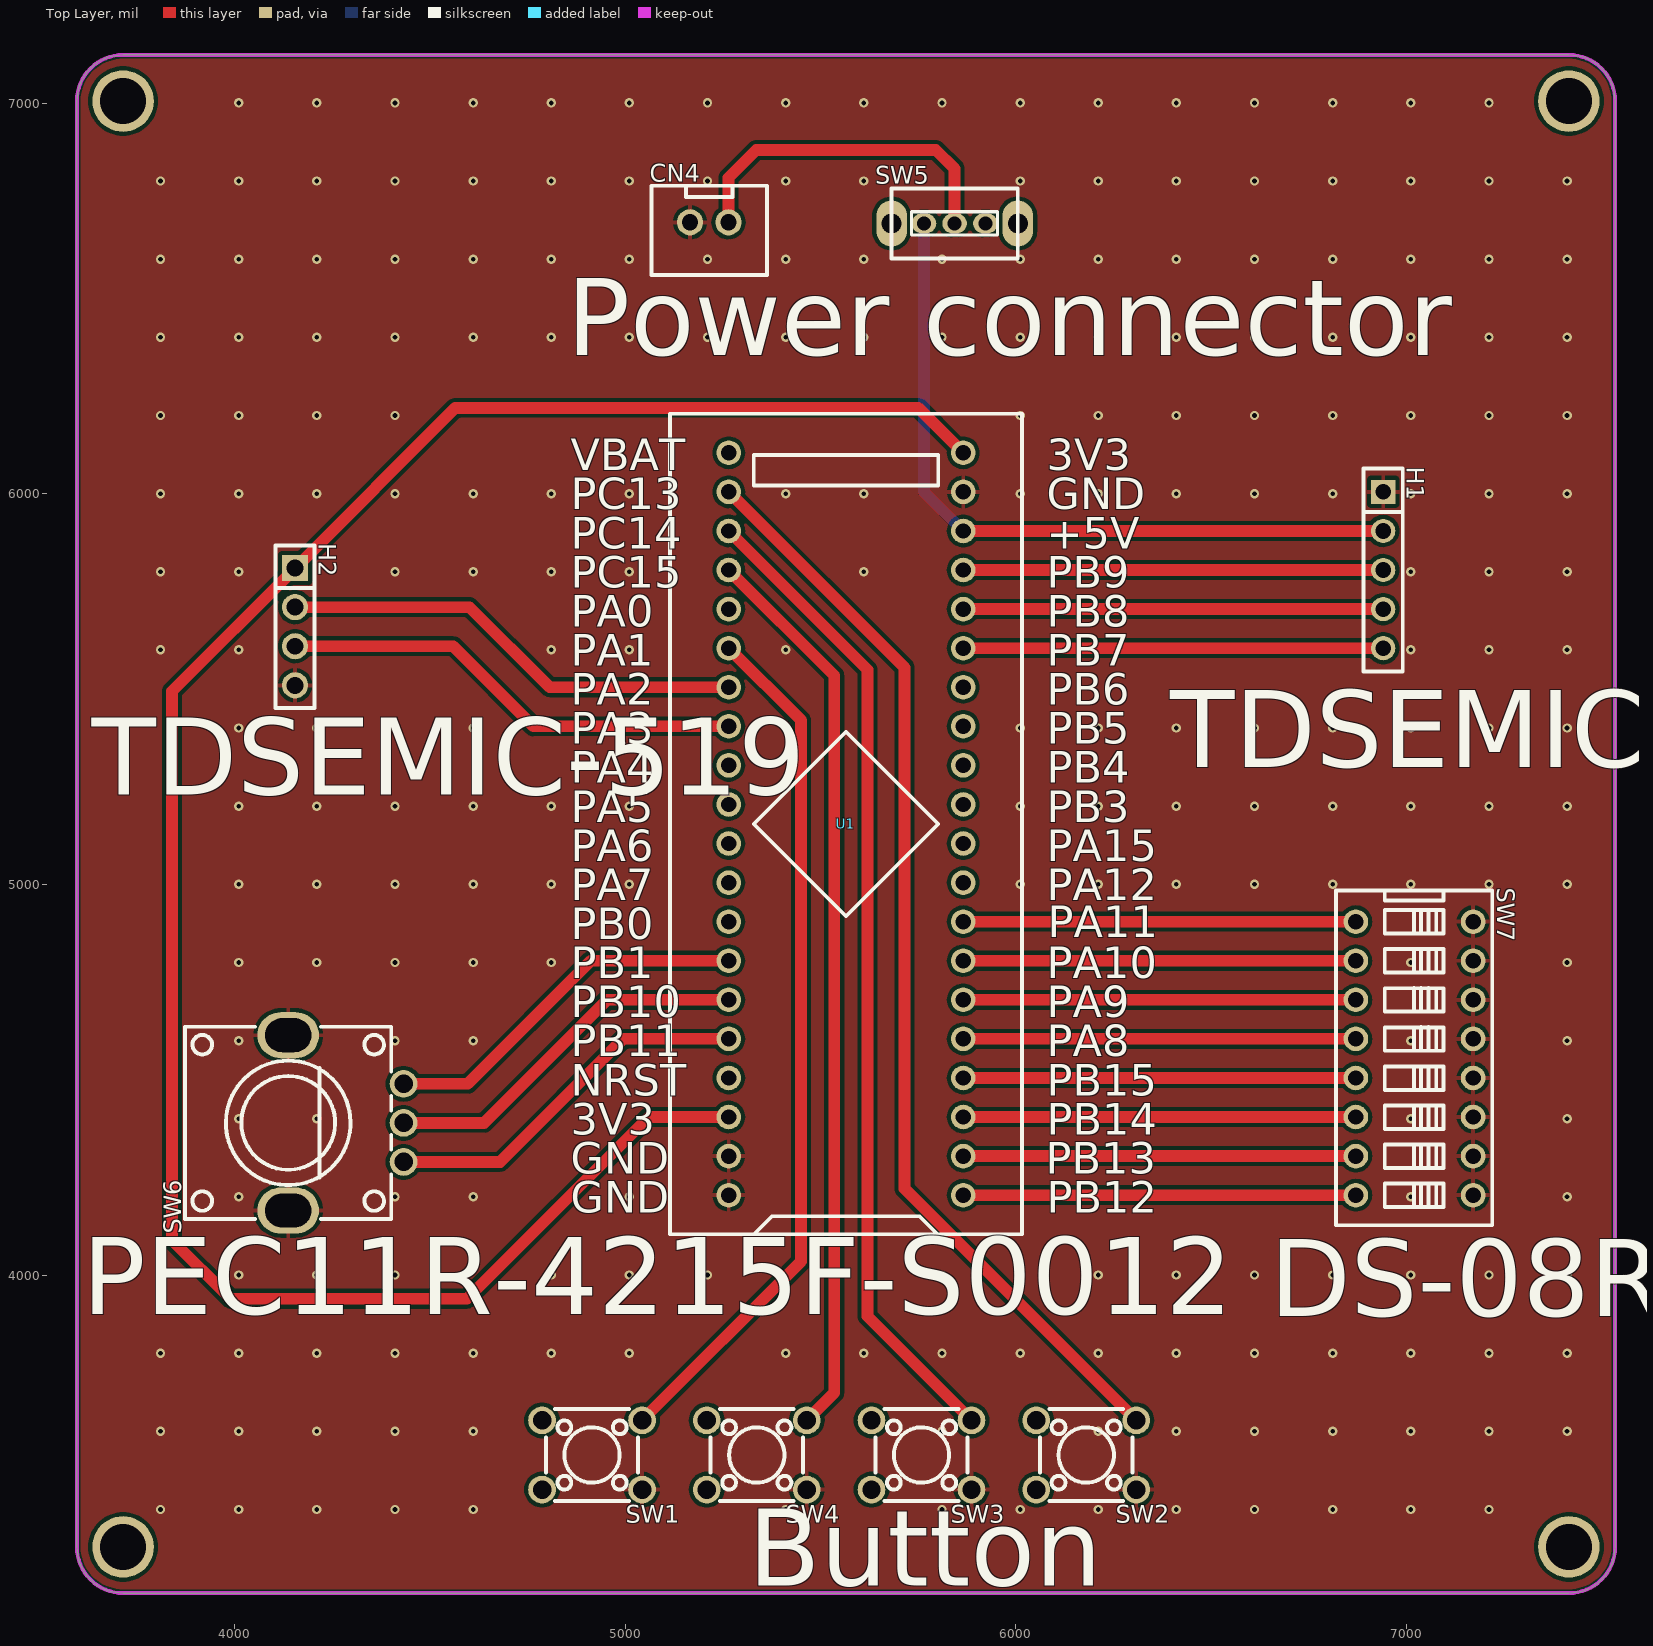
[diagram p0: Top Layer view]
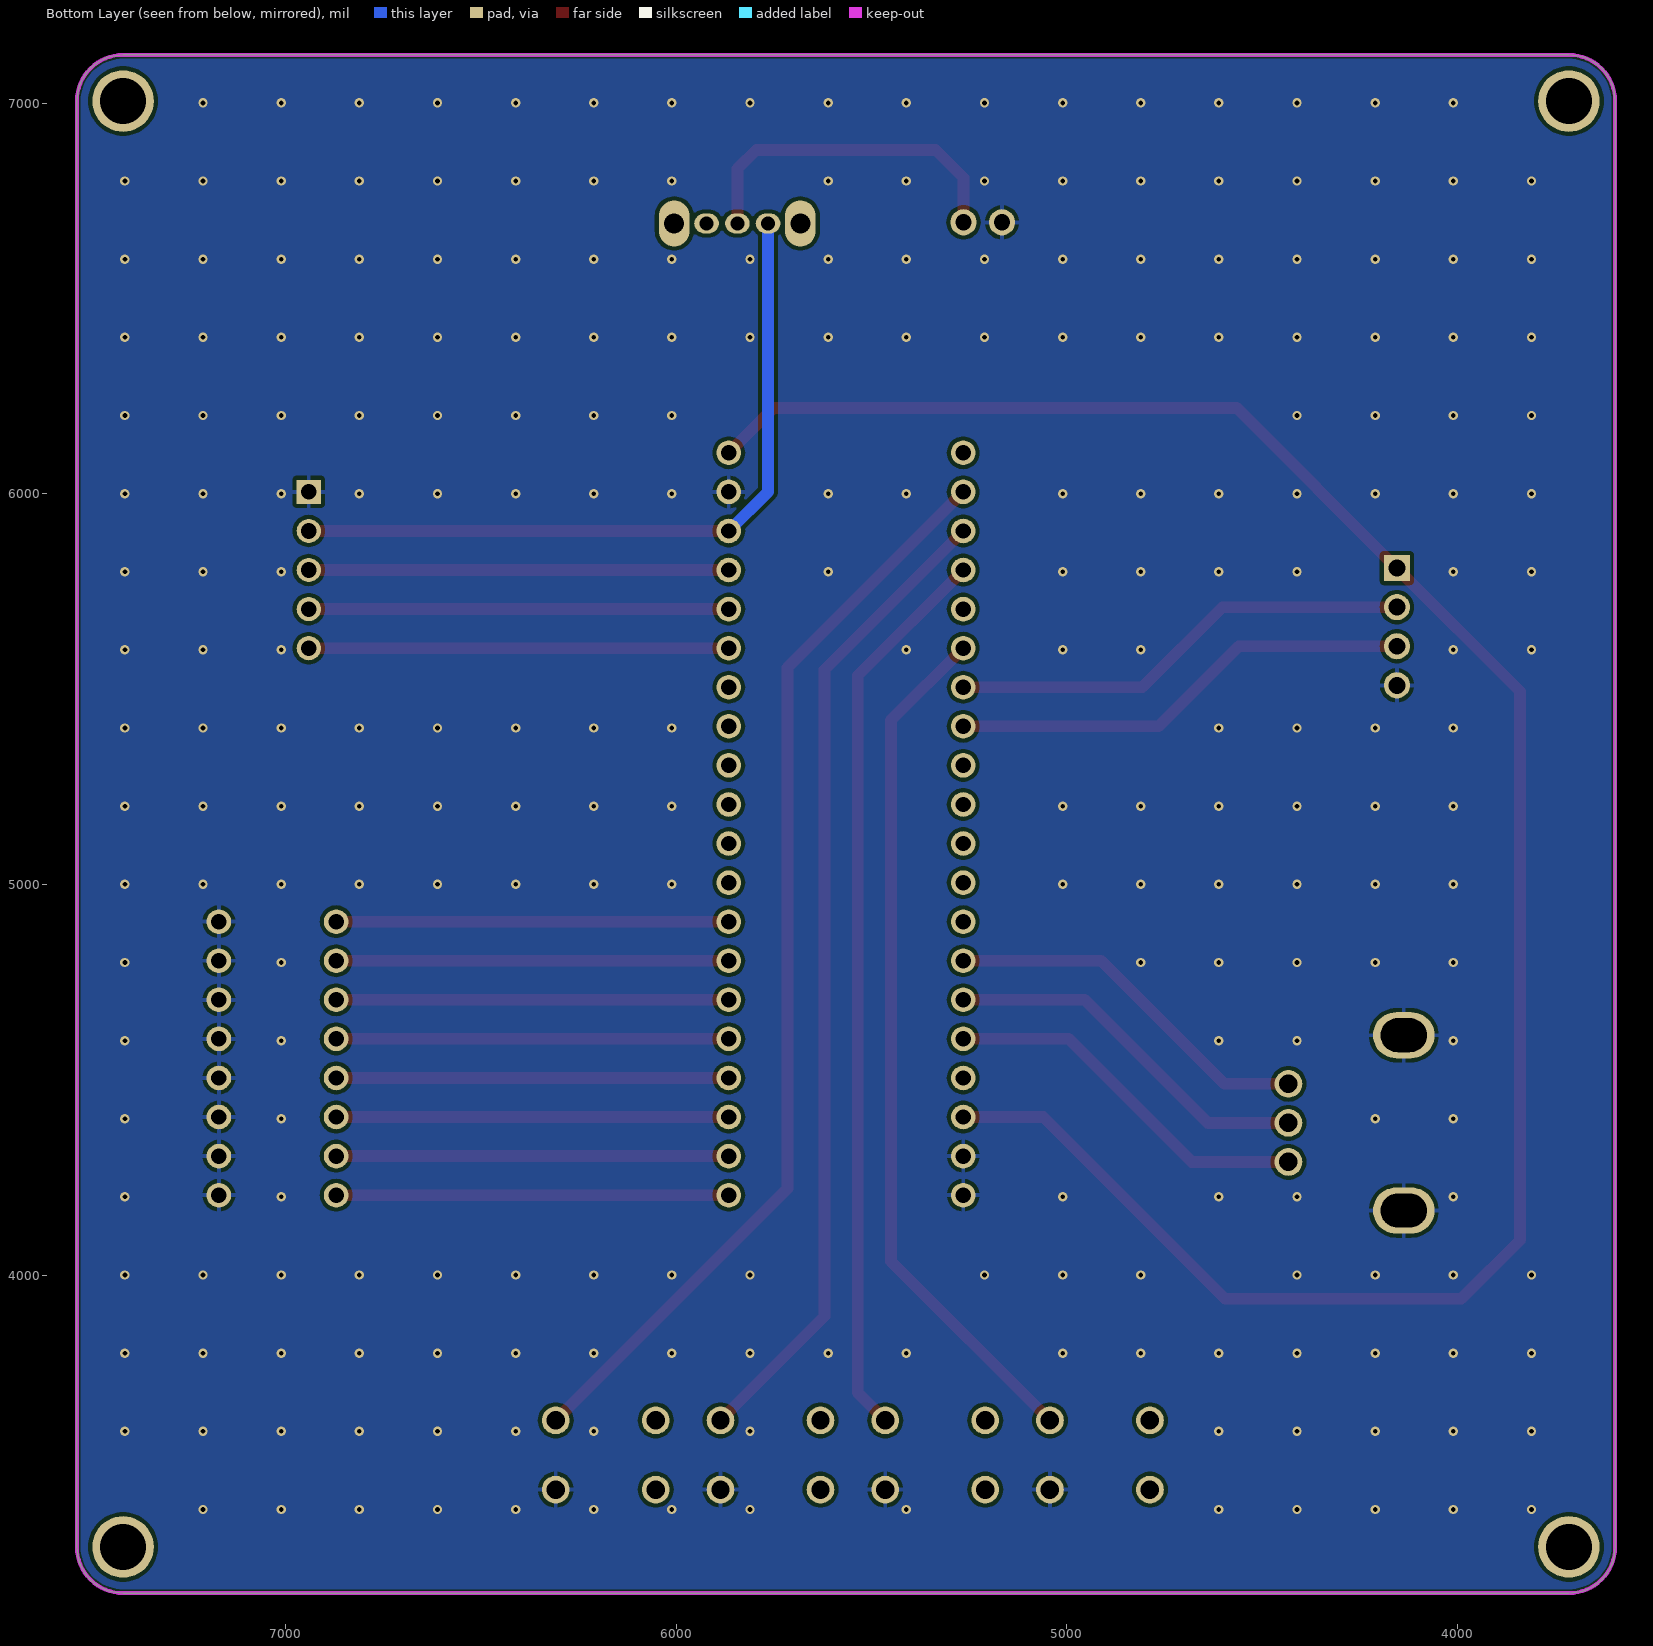
[diagram p1: Bottom Layer view, seen from below]
# Altium PCB MISC51872.pcbdoc
Units mil, origin at the board's own origin, x right, y up, seen from the top; angles counter-clockwise.
Board outline 3937.01 x 3937.01 mil, 2 copper layers (Top Layer, Bottom Layer), stack 62.206 mil thick; 11 components, 38 nets, 97 pads, 243 vias.

## Layer stack, top to bottom
Top Solder Mask Layer: solder mask 0.394, Dk 3.3
Top Layer: signal copper 1.379
Dielectric1: surface 59.449, FR4, Dk 4.5
Bottom Layer: signal copper 1.378
Bottom Solder Mask Layer: solder mask 0.394, Dk 3.3

## Board outline
3714.61,7123.5 ccw(c3714.61,7005.39) 3596.5,7005.39 3596.5,3304.61 ccw(c3714.61,3304.61) 3714.61,3186.5 7415.39,3186.5 ccw(c7415.39,3304.61) 7533.5,3304.61 7533.5,7005.39 ccw(c7415.39,7005.39) 7415.39,7123.5 3714.61,7123.5

## Design rules (kind name [scope] priority, off if disabled: settings)
BoardOutlineClearance copperThickness2oz_1 [All] p2 off: genericclearance=7.99 ignorepadtopadclearanceinfootprint=FALSE except(0: Arc-SplitContinuation Track-SplitContinuation SMDPad-SplitContinuation THPad-SplitContinuation Via-SplitContinuation Fill-SplitContinuation Region-SplitContinuation Poly-SplitContinuation Text-SplitContinuation Hole-SplitContinuation; 5.98: Arc-CutoutEdge Track-CutoutEdge SMDPad-CutoutEdge THPad-CutoutEdge Via-CutoutEdge Text-CutoutEdge; 6.9: Hole-OutlineEdge Hole-CutoutEdge; 10: Poly-OutlineEdge Poly-CutoutEdge; 11.81: Arc-OutlineEdge Track-OutlineEdge SMDPad-OutlineEdge THPad-OutlineEdge Via-OutlineEdge Fill-OutlineEdge Region-OutlineEdge Text-OutlineEdge Fill-CutoutEdge Region-CutoutEdge)
BoardOutlineClearance Plane_innerPlane_1 [All] p4 off: genericclearance=4.02 ignorepadtopadclearanceinfootprint=FALSE except(0: Arc-SplitContinuation Track-SplitContinuation SMDPad-SplitContinuation THPad-SplitContinuation Via-SplitContinuation Fill-SplitContinuation Region-SplitContinuation Poly-SplitContinuation Text-SplitContinuation Hole-SplitContinuation; 5.98: Arc-CutoutEdge Track-CutoutEdge SMDPad-CutoutEdge THPad-CutoutEdge Via-CutoutEdge Text-CutoutEdge; 6.9: Hole-OutlineEdge Hole-CutoutEdge; 10: Poly-OutlineEdge Poly-CutoutEdge; 11.81: Arc-OutlineEdge Track-OutlineEdge SMDPad-OutlineEdge THPad-OutlineEdge Via-OutlineEdge Fill-OutlineEdge Region-OutlineEdge Text-OutlineEdge Fill-CutoutEdge Region-CutoutEdge)
BoardOutlineClearance Copper_copperRegion_1 [All] p6 off: genericclearance=4.02 ignorepadtopadclearanceinfootprint=FALSE except(0: Arc-SplitContinuation Track-SplitContinuation SMDPad-SplitContinuation THPad-SplitContinuation Via-SplitContinuation Fill-SplitContinuation Region-SplitContinuation Poly-SplitContinuation Text-SplitContinuation Hole-SplitContinuation; 5.98: Arc-CutoutEdge Track-CutoutEdge SMDPad-CutoutEdge THPad-CutoutEdge Via-CutoutEdge Text-CutoutEdge; 6.9: Hole-OutlineEdge Hole-CutoutEdge; 10: Poly-OutlineEdge Poly-CutoutEdge; 11.81: Arc-OutlineEdge Track-OutlineEdge SMDPad-OutlineEdge THPad-OutlineEdge Via-OutlineEdge Fill-OutlineEdge Region-OutlineEdge Text-OutlineEdge Fill-CutoutEdge Region-CutoutEdge)
BoardOutlineClearance copperThickness1oz_1 [All] p8: genericclearance=4.02 ignorepadtopadclearanceinfootprint=FALSE except(0: Arc-SplitContinuation Track-SplitContinuation SMDPad-SplitContinuation THPad-SplitContinuation Via-SplitContinuation Fill-SplitContinuation Region-SplitContinuation Poly-SplitContinuation Text-SplitContinuation Hole-SplitContinuation; 5.98: Arc-CutoutEdge Track-CutoutEdge SMDPad-CutoutEdge THPad-CutoutEdge Via-CutoutEdge Text-CutoutEdge; 6.9: Hole-OutlineEdge Hole-CutoutEdge; 10: Poly-OutlineEdge Poly-CutoutEdge; 11.81: Arc-OutlineEdge Track-OutlineEdge SMDPad-OutlineEdge THPad-OutlineEdge Via-OutlineEdge Fill-OutlineEdge Region-OutlineEdge Text-OutlineEdge Fill-CutoutEdge Region-CutoutEdge)
Clearance copperThickness2oz [All] p1 off: gap=7.99 ignorepadtopadclearanceinfootprint=FALSE except(5.98: SMDPad-Track SMDPad-SMDPad THPad-Track SMDPad-THPad THPad-THPad Track-Via SMDPad-Via THPad-Via Via-Via Fill-SMDPad Region-SMDPad Fill-THPad Region-THPad Fill-Via Region-Via Fill-Fill Fill-Region Region-Region Arc-Track Arc-SMDPad Arc-THPad Arc-Via Fill-Arc Region-Arc Arc-Arc Text-Track SMDPad-Text Text-THPad Text-Via Fill-Text Region-Text Arc-Text Text-Text; 6.9: Hole-Track Hole-SMDPad Hole-THPad Hole-Via Fill-Hole Region-Hole Hole-Arc Hole-Text; 10: Poly-Track Poly-SMDPad Poly-THPad Poly-Via Poly-Fill Poly-Region Poly-Poly Poly-Arc Poly-Text Poly-Hole; 11.81: Fill-Track Region-Track)
Clearance Plane_innerPlane [All] p3 off: gap=4.02 ignorepadtopadclearanceinfootprint=FALSE except(5.98: SMDPad-Track SMDPad-SMDPad THPad-Track SMDPad-THPad THPad-THPad Track-Via SMDPad-Via THPad-Via Via-Via Fill-SMDPad Region-SMDPad Fill-THPad Region-THPad Fill-Via Region-Via Fill-Fill Fill-Region Region-Region Arc-Track Arc-SMDPad Arc-THPad Arc-Via Fill-Arc Region-Arc Arc-Arc Text-Track SMDPad-Text Text-THPad Text-Via Fill-Text Region-Text Arc-Text Text-Text; 6.9: Hole-Track Hole-SMDPad Hole-THPad Hole-Via Fill-Hole Region-Hole Hole-Arc Hole-Text; 10: Poly-Track Poly-SMDPad Poly-THPad Poly-Via Poly-Fill Poly-Region Poly-Poly Poly-Arc Poly-Text Poly-Hole; 11.81: Fill-Track Region-Track)
Clearance Copper_copperRegion [All] p5 off: gap=4.02 ignorepadtopadclearanceinfootprint=FALSE except(5.98: SMDPad-Track SMDPad-SMDPad THPad-Track SMDPad-THPad THPad-THPad Track-Via SMDPad-Via THPad-Via Via-Via Fill-SMDPad Region-SMDPad Fill-THPad Region-THPad Fill-Via Region-Via Fill-Fill Fill-Region Region-Region Arc-Track Arc-SMDPad Arc-THPad Arc-Via Fill-Arc Region-Arc Arc-Arc Text-Track SMDPad-Text Text-THPad Text-Via Fill-Text Region-Text Arc-Text Text-Text; 6.9: Hole-Track Hole-SMDPad Hole-THPad Hole-Via Fill-Hole Region-Hole Hole-Arc Hole-Text; 10: Poly-Track Poly-SMDPad Poly-THPad Poly-Via Poly-Fill Poly-Region Poly-Poly Poly-Arc Poly-Text Poly-Hole; 11.81: Fill-Track Region-Track)
Clearance copperThickness1oz [All] p7: gap=4.02 ignorepadtopadclearanceinfootprint=FALSE except(5.98: SMDPad-Track SMDPad-SMDPad THPad-Track SMDPad-THPad THPad-THPad Track-Via SMDPad-Via THPad-Via Via-Via Fill-SMDPad Region-SMDPad Fill-THPad Region-THPad Fill-Via Region-Via Fill-Fill Fill-Region Region-Region Arc-Track Arc-SMDPad Arc-THPad Arc-Via Fill-Arc Region-Arc Arc-Arc Text-Track SMDPad-Text Text-THPad Text-Via Fill-Text Region-Text Arc-Text Text-Text; 6.9: Hole-Track Hole-SMDPad Hole-THPad Hole-Via Fill-Hole Region-Hole Hole-Arc Hole-Text; 10: Poly-Track Poly-SMDPad Poly-THPad Poly-Via Poly-Fill Poly-Region Poly-Poly Poly-Arc Poly-Text Poly-Hole; 11.81: Fill-Track Region-Track)
DiffPairsRouting differentialPair [All] p1: maxlimit=6 minlimit=6 mostfreqgap=6 toplayer_minwidth=5 toplayer_prefwidth=10 toplayer_maxwidth=100 toplayer_mingap=6 toplayer_prefgap=6 toplayer_maxgap=6 bottomlayer_minwidth=5 bottomlayer_prefwidth=10 bottomlayer_maxwidth=100 bottomlayer_mingap=6 bottomlayer_prefgap=6 bottomlayer_maxgap=6 maxuncoupledlength=10
HoleToHoleClearance otherClearance [All] p1: gap=11.81 allowstackedmicrovias=TRUE
Length netLength [All] p1: minlimit=0 maxlimit=0
PasteMaskExpansion pasteMaskExpansion [All] p1: expansion=0
PlaneConnect innerPlane [All] p1: planeconnectstyle=Relief reliefexpansion=20 reliefentries=4 reliefconductorwidth=10 reliefairgap=10
PolygonConnect copperRegion [All] p1: connectstyle=Relief reliefconductorwidth=10 reliefentries=4 polygonreliefangle="90 Angle" airgapwidth=10 via.connectstyle=Relief via.reliefconductorwidth=10 via.reliefentries=4 via.polygonreliefangle="90 Angle" via.airgapwidth=10
RoutingVias viaSize [All] p1: holewidth=12.01 width=24.02 viastyle="Through Hole" minholewidth=11.81 minwidth=19.68 maxholewidth=248.03 maxwidth=393.7
SolderMaskExpansion solderMaskExpansion [IsVia] p1: expansion=-1000 istentingtop=TRUE
SolderMaskExpansion solderMaskExpansion [All] p2: expansion=2 istentingtop=FALSE
Width copperThickness2oz_2 [All] p1 off: maxlimit=100 minlimit=8 preferedwidth=10
Width copperThickness1oz_2 [All] p2: maxlimit=100 minlimit=5 preferedwidth=10

## Components (designator, comment, footprint, x,y, rotation, side; value= is the part's Value field where it differs from the comment)
CN4 "XH2.54*2P_THT" CONN-TH_2P-P2.50-XH2.54-2P 5215,6695 r0 top
H1 "" HDR-TH_5P-P2.54-V-F 6940,5805 r270 top
H2 "" HDR-TH_4P-P2.54-V-F 4155,5660 r270 top
SW1 "" SW-TH_4P-L6.0-W6.0-P4.50-LS6.5 4915,3540 r180 top
SW2 "" SW-TH_4P-L6.0-W6.0-P4.50-LS6.5 6179.9,3540 r180 top
SW3 "" SW-TH_4P-L6.0-W6.0-P4.50-LS6.5 5758.27,3540 r180 top
SW4 "" SW-TH_4P-L6.0-W6.0-P4.50-LS6.5 5336.63,3540 r180 top
SW5 "" 拨动开关 5837.9,6692.05 r0 top
SW6 "PEC11R-4215F-N0024" SW-TH_PEC11R-4215F-N0024 4285,4390 r90 top
SW7 "DS-08RP" SW-TH_DS-08XP 7020,4555 r270 top
U1 "STM32F103C8T6-Card" CONN-TH_L53.3-W22.9_STM32F103C8T6-CARD 5565,5155 r90 top

## Footprints (in the part's own frame and the unit in brackets; to place one, negate y for a bottom-side part, rotate by r counter-clockwise, add the part's x,y. Pads: shape width x height; smd on the part's side, far side on the other; paste and mask are expansions set on the pad)
CONN-TH_2P-P2.50-XH2.54-2P [mm]
  round 1.7 hole 1.05 paste+0 mask+0.05: 1(1.25,0) 2(-1.25,0)
  silkscreen extent -3.75,-3.42 3.75,2.37
CONN-TH_L53.3-W22.9_STM32F103C8T6-CARD [mm]
  round 1.6 hole 1: 1(-24.13,-7.62) 2(-21.59,-7.62) 3(-19.05,-7.62) 4(-16.51,-7.62) 5(-13.97,-7.62) 6(-11.43,-7.62) 7(-8.89,-7.62) 8(-6.35,-7.62) 9(-3.81,-7.62) 10(-1.27,-7.62) 11(1.27,-7.62) 12(3.81,-7.62) 13(6.35,-7.62) 14(8.89,-7.62) 15(11.43,-7.62) 16(13.97,-7.62) 17(16.51,-7.62) 18(19.05,-7.62) 19(21.59,-7.62) 20(24.13,-7.62) 21(24.13,7.62) 22(21.59,7.62) 23(19.05,7.62) 24(16.51,7.62) 25(13.97,7.62) 26(11.43,7.62) 27(8.89,7.62) 28(6.35,7.62) 29(3.81,7.62) 30(1.27,7.62) 31(-1.27,7.62) 32(-3.81,7.62) 33(-6.35,7.62) 34(-8.89,7.62) 35(-11.43,7.62) 36(-13.97,7.62) 37(-16.51,7.62) 38(-19.05,7.62) 39(-21.59,7.62) 40(-24.13,7.62)
  silkscreen extent -26.67,-11.43 26.67,11.43
HDR-TH_4P-P2.54-V-F [mm]
  rect 1.7x1.7 hole 1.1: 1(-3.81,0)
  round 1.7 hole 1.1: 2(-1.27,0) 3(1.27,0) 4(3.81,0)
  silkscreen extent -5.29,-1.27 5.29,1.27
HDR-TH_5P-P2.54-V-F [mil]
  rect 62x62 hole 40.16: 1(-200,0)
  round 62 hole 40.16: 2(-100,0) 3(0,0) 4(100,0) 5(200,0)
  silkscreen extent -260,-50 260,50
SW-TH_4P-L6.0-W6.0-P4.50-LS6.5 [mm]
  round 1.8 hole 1.2: 1(-3.25,2.25) 2(3.25,2.25) 3(-3.25,-2.25) 4(3.25,-2.25)
  silkscreen extent -3,-3 3,3
SW-TH_DS-08XP [mm]
  round 1.6 hole 1: 1(-8.89,3.81) 2(-6.35,3.81) 3(-3.81,3.81) 4(-1.27,3.81) 5(1.27,3.81) 6(3.81,3.81) 7(6.35,3.81) 8(8.89,3.81) 9(8.89,-3.81) 10(6.35,-3.81) 11(3.81,-3.81) 12(1.27,-3.81) 13(-1.27,-3.81) 14(-3.81,-3.81) 15(-6.35,-3.81) 16(-8.89,-3.81)
  silkscreen extent -10.91,-5.11 10.85,5.05
SW-TH_PEC11R-4215F-N0024 [mm]
  oval 3x4 hole 2.2 slot 3 at 90 deg: 4(-5.7,3.75) 5(5.7,3.75)
  round 1.8 hole 1.2: A(-2.54,-3.75) B(2.54,-3.75) C(0,-3.75)
  silkscreen extent -6.25,-2.95 6.25,10.45
拨动开关 [mil]
  oval 63x51.2 hole 35.4 paste+0 mask+2: 1(-73.4,0) 2(5,0) 3(84,0)
  oval 78.7x118.1 hole 51.2 paste+0 mask+2: 4(166.7,0) 5(-156.1,0)
  silkscreen extent -156,-90 167,90

## Free pads (board coordinates)
  round 157.48 hole 118.11: 1(3714.61,7005.39) 1(3714.61,3304.61) 1(7415.39,7005.39) 1(7415.39,3304.61)

## Via types
v1: diameter 24.02, hole 12, Top Layer to Bottom Layer, 243 vias

## Nets (pads, with @x,y where several pads share a name; then routed paths per layer and width w, separated by ;. In a path a pad name is that pad's centre, name@x,y a point inside that pad or via, vN(x,y) a via of type N, cw(c..) or ccw(c..) an arc to the next point about the centre after c; other vN are vias at no path point)
$1N17118: CN4.1 SW5.2 | length 882.1
  Top Layer w30: CN4.1 5264.22,6809.22 5335,6880 5795,6880 5842.9,6832.1 SW5.2
+5V: H1.2 SW5.1 U1.18 | length 1903.7
  Top Layer w30: U1.18 H1.2
  Bottom Layer w30: SW5.1 5764.5,6005.5 U1.18
GND: CN4.2 H1.1 H2.4 SW1.1 SW2.1 SW3.1 SW4.1 SW6.4 SW6.5 SW7.1 SW7.2 SW7.3 SW7.4 SW7.5 SW7.6 SW7.7 SW7.8 U1.19 U1.39 U1.40
  other v1: 3810.6,3400.6 4010.6,3400.6 4210.6,3400.6 4410.6,3400.6 4610.6,3400.6 5410.6,3400.6 5810.6,3400.6 6010.6,3400.6 6210.6,3400.6 6410.6,3400.6 6610.6,3400.6 6810.6,3400.6 7010.6,3400.6 7210.6,3400.6 3810.6,3600.6 4010.6,3600.6 4210.6,3600.6 4410.6,3600.6 4610.6,3600.6 5810.6,3600.6 6210.6,3600.6 6410.6,3600.6 6610.6,3600.6 6810.6,3600.6 7010.6,3600.6 7210.6,3600.6 7410.6,3600.6 3810.6,3800.6 4010.6,3800.6 4210.6,3800.6 4410.6,3800.6 4610.6,3800.6 4810.6,3800.6 5010.6,3800.6 5410.6,3800.6 5610.6,3800.6 5810.6,3800.6 6010.6,3800.6 6210.6,3800.6 6410.6,3800.6 6610.6,3800.6 6810.6,3800.6 7010.6,3800.6 7210.6,3800.6 7410.6,3800.6 3810.6,4000.6 4010.6,4000.6 4210.6,4000.6 4410.6,4000.6 4810.6,4000.6 5010.6,4000.6 5210.6,4000.6 5810.6,4000.6 6010.6,4000.6 6210.6,4000.6 6410.6,4000.6 6610.6,4000.6 6810.6,4000.6 7010.6,4000.6 7210.6,4000.6 7410.6,4000.6 4010.6,4200.6 4410.6,4200.6 4610.6,4200.6 5010.6,4200.6 7010.6,4200.6 7410.6,4200.6 4010.6,4400.6 4210.6,4400.6 7010.6,4400.6 7410.6,4400.6 4010.6,4600.6 4410.6,4600.6 4610.6,4600.6 7010.6,4600.6 7410.6,4600.6 4010.6,4800.6 4210.6,4800.6 4410.6,4800.6 4610.6,4800.6 4810.6,4800.6 7010.6,4800.6 7410.6,4800.6 4010.6,5000.6 4210.6,5000.6 4410.6,5000.6 4610.6,5000.6 4810.6,5000.6 5010.6,5000.6 6010.6,5000.6 6210.6,5000.6 6410.6,5000.6 6610.6,5000.6 6810.6,5000.6 7010.6,5000.6 7210.6,5000.6 7410.6,5000.6 4010.6,5200.6 4210.6,5200.6 4410.6,5200.6 4610.6,5200.6 4810.6,5200.6 5010.6,5200.6 6010.6,5200.6 6210.6,5200.6 6410.6,5200.6 6610.6,5200.6 6810.6,5200.6 7010.6,5200.6 7210.6,5200.6 7410.6,5200.6 4010.6,5400.6 4210.6,5400.6 4410.6,5400.6 4610.6,5400.6 6010.6,5400.6 6210.6,5400.6 6410.6,5400.6 6610.6,5400.6 6810.6,5400.6 7010.6,5400.6 7210.6,5400.6 7410.6,5400.6 3810.6,5600.6 4010.6,5600.6 4810.6,5600.6 5010.6,5600.6 5410.6,5600.6 7010.6,5600.6 7210.6,5600.6 7410.6,5600.6 3810.6,5800.6 4010.6,5800.6 4410.6,5800.6 4610.6,5800.6 4810.6,5800.6 5010.6,5800.6 5610.6,5800.6 7010.6,5800.6 7210.6,5800.6 7410.6,5800.6 3810.6,6000.6 4010.6,6000.6 4210.6,6000.6 4410.6,6000.6 4610.6,6000.6 4810.6,6000.6 5010.6,6000.6 5410.6,6000.6 5610.6,6000.6 6010.6,6000.6 6210.6,6000.6 6410.6,6000.6 6610.6,6000.6 6810.6,6000.6 7010.6,6000.6 7210.6,6000.6 7410.6,6000.6 3810.6,6200.6 4010.6,6200.6 4210.6,6200.6 4410.6,6200.6 6010.6,6200.6 6210.6,6200.6 6410.6,6200.6 6610.6,6200.6 6810.6,6200.6 7010.6,6200.6 7210.6,6200.6 7410.6,6200.6 3810.6,6400.6 4010.6,6400.6 4210.6,6400.6 4410.6,6400.6 4610.6,6400.6 4810.6,6400.6 5010.6,6400.6 5210.6,6400.6 5410.6,6400.6 5610.6,6400.6 5810.6,6400.6 6010.6,6400.6 6210.6,6400.6 6410.6,6400.6 6610.6,6400.6 6810.6,6400.6 7010.6,6400.6 7210.6,6400.6 7410.6,6400.6 3810.6,6600.6 4010.6,6600.6 4210.6,6600.6 4410.6,6600.6 4610.6,6600.6 4810.6,6600.6 5010.6,6600.6 5210.6,6600.6 5410.6,6600.6 5610.6,6600.6 5810.6,6600.6 6010.6,6600.6 6210.6,6600.6 6410.6,6600.6 6610.6,6600.6 6810.6,6600.6 7010.6,6600.6 7210.6,6600.6 7410.6,6600.6 3810.6,6800.6 4010.6,6800.6 4210.6,6800.6 4410.6,6800.6 4610.6,6800.6 4810.6,6800.6 5010.6,6800.6 5210.6,6800.6 5410.6,6800.6 5610.6,6800.6 6010.6,6800.6 6210.6,6800.6 6410.6,6800.6 6610.6,6800.6 6810.6,6800.6 7010.6,6800.6 7210.6,6800.6 7410.6,6800.6 4010.6,7000.6 4210.6,7000.6 4410.6,7000.6 4610.6,7000.6 4810.6,7000.6 5010.6,7000.6 5210.6,7000.6 5410.6,7000.6 5610.6,7000.6 5810.6,7000.6 6010.6,7000.6 6210.6,7000.6 6410.6,7000.6 6610.6,7000.6 6810.6,7000.6 7010.6,7000.6 7210.6,7000.6
NRST: U1.37
PA0: U1.25
PA1: SW1.3 U1.26 | length 2221.7
  Top Layer w30: SW1.3 5450,4035.63 5450,5420 U1.26
PA2: H2.2 U1.27 | length 1194.9
  Top Layer w30: H2.2 4601.42,5710 4806.42,5505 U1.27
PA3: H2.3 U1.28 | length 1194.9
  Top Layer w30: H2.3 4560,5610 4765,5405 U1.28
PA4: U1.29
PA5: U1.30
PA6: U1.31
PA7: U1.32
PA8: SW7.13 U1.5 | length 1005
  Top Layer w30: U1.5 SW7.13
PA9: SW7.14 U1.6 | length 1005
  Top Layer w30: U1.6 SW7.14
PA10: SW7.15 U1.7 | length 1005
  Top Layer w30: U1.7 SW7.15
PA11: SW7.16 U1.8 | length 1005
  Top Layer w30: U1.8 SW7.16
PA12: U1.9
PA15: U1.10
PB0: U1.33
PB1: SW6.B U1.34 | length 962.8
  Top Layer w30: SW6.B 4597.16,4490 4912.16,4805 U1.34
PB3: U1.11
PB4: U1.12
PB5: U1.13
PB6: U1.14
PB7: H1.5 U1.15 | length 1075
  Top Layer w30: U1.15 H1.5
PB8: H1.4 U1.16 | length 1075
  Top Layer w30: U1.16 H1.4
PB9: H1.3 U1.17 | length 1075
  Top Layer w30: U1.17 H1.3
PB10: SW6.C U1.35 | length 962.8
  Top Layer w30: SW6.C 4638.58,4390 4953.58,4705 U1.35
PB11: SW6.A U1.36 | length 962.8
  Top Layer w30: SW6.A 4680,4290 4995,4605 U1.36
PB12: SW7.9 U1.1 | length 1005
  Top Layer w30: U1.1 SW7.9
PB13: SW7.10 U1.2 | length 1005
  Top Layer w30: U1.2 SW7.10
PB14: SW7.11 U1.3 | length 1005
  Top Layer w30: U1.3 SW7.11
PB15: SW7.12 U1.4 | length 1005
  Top Layer w30: U1.4 SW7.12
PC13: SW2.3 U1.22 | length 2808.4
  Top Layer w30: U1.22 5715,5555 5715,4221.43 SW2.3@6307.85,3628.58
PC14: SW3.3 U1.23 | length 2533.7
  Top Layer w30: U1.23 5620,5550 5620,3894.8 SW3.3
PC15: SW4.3 U1.24 | length 2317.4
  Top Layer w30: U1.24 5535,5535 5535,3699 SW4.3
VBAT: U1.21
VCC: H2.1 U1.20 U1.38 | length 5457.7
  Top Layer w30: U1.38 5060,4405 4595,3940 3990,3940 3840,4090 3840,5495 H2.1 4565,6220 5750,6220 U1.20
pads on no net: SW1.2 SW1.4 SW2.2 SW2.4 SW3.2 SW3.4 SW4.2 SW4.4 SW5.3 SW5.4 SW5.5

## Polygon pours and split planes (outlines as drawn)
GND on Bottom Layer (solid, remove dead copper, pour order 4): 3525,7245 3525,3080 7700,3080 7700,7245
GND on Top Layer (solid, remove dead copper, pour order 2): 3000,7415 3000,3000 7930,3000 7930,7415
GND on Top Layer (solid, remove dead copper, pour order 4): 3395,7205 3395,3035 7995,3035 7995,7205

## Keep-outs
Board Outline Layer:
  the board outline again, w10

## Silkscreen, mask and mechanical layers (free items; w line width, h text height)
Top Silkscreen Layer:
  text "Power connector" at 4850,6355 h196.85
  text "VBAT" at 4860.95,6060 h80
  text "3V3" at 6079.16,6060 h80
  text "PC13" at 4860.95,5960 h80
  text "GND" at 6079.16,5960 h80
  text "PC14" at 4860.95,5860 h80
  text "+5V" at 6079.16,5860 h80
  text "PC15" at 4860.95,5760 h80
  text "PB9" at 6079.16,5760 h80
  text "PA0" at 4860.95,5660 h80
  text "PB8" at 6079.16,5660 h80
  text "PA1" at 4860.95,5560 h80
  text "PB7" at 6079.16,5560 h80
  text "PA2" at 4860.95,5460 h80
  text "PB6" at 6079.16,5460 h80
  text "PA3" at 4860.95,5360 h80
  text "PB5" at 6079.16,5360 h80
  text "TDSEMIC-504" at 6395,5300 h196.85
  text "PA4" at 4860.95,5260 h80
  text "PB4" at 6079.16,5260 h80
  text "TDSEMIC-519" at 3635,5230 h196.85
  text "PA5" at 4860.95,5160 h80
  text "PB3" at 6079.16,5160 h80
  text "PA6" at 4860.95,5060 h80
  text "PA15" at 6079.16,5060 h80
  text "PA7" at 4860.95,4960 h80
  text "PA12" at 6079.16,4960 h80
  text "PA11" at 6080.95,4865 h80
  text "PB0" at 4860.95,4860 h80
  text "PB1" at 4860.95,4760 h80
  text "PA10" at 6079.16,4760 h80
  text "PB10" at 4860.95,4660 h80
  text "PA9" at 6079.16,4660 h80
  text "PB11" at 4860.95,4560 h80
  text "PA8" at 6079.16,4560 h80
  text "NRST" at 4860.95,4460 h80
  text "PB15" at 6079.16,4460 h80
  text "3V3" at 4860.95,4360 h80
  text "PB14" at 6079.16,4360 h80
  text "GND" at 4860.95,4260 h80
  text "PB13" at 6075.95,4260 h80
  text "GND" at 4860.95,4160 h80
  text "PB12" at 6079.16,4160 h80
  text "PEC11R-4215F-S0012" at 3610,3900 h196.85
  text "DS-08RP" at 6650,3895 h196.85
  text "Button" at 5315,3205 h196.85